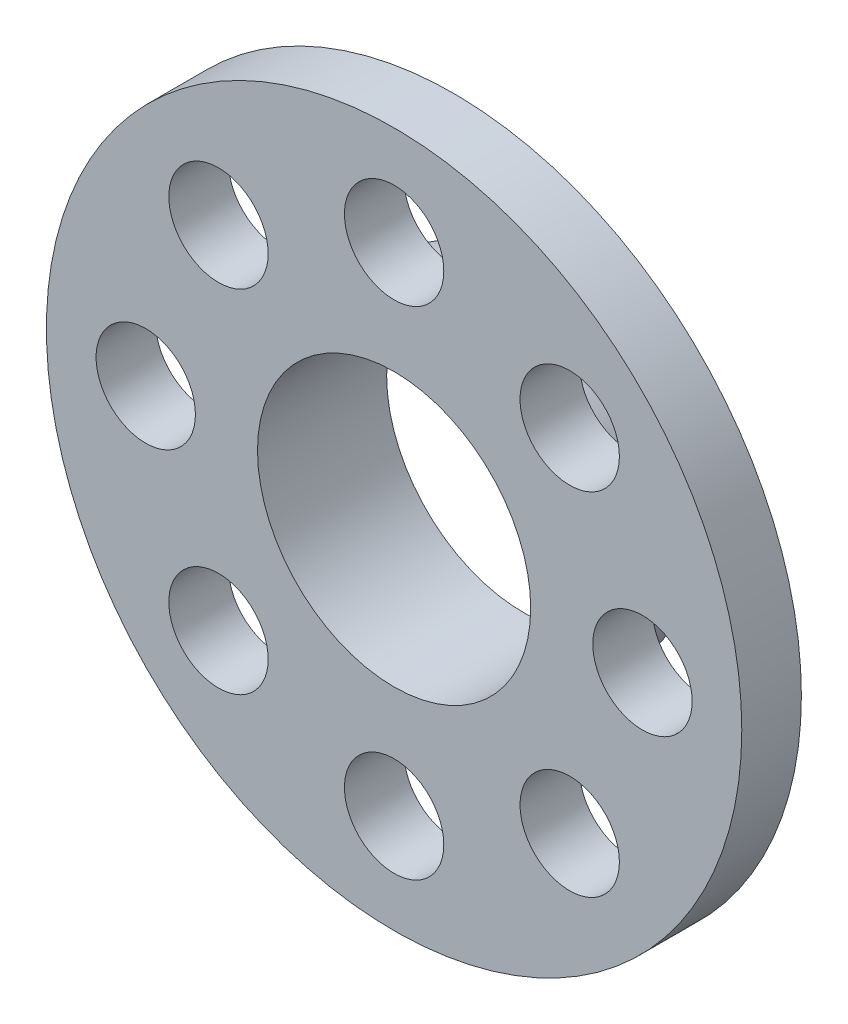
SolidWorks part; units mm, degrees
ref_plane "Front Plane" through (0, 0, 0) normal (0, 0, 1) x (1, 0, 0)
ref_plane "Top Plane" through (0, 0, 0) normal (0, 1, 0) x (1, 0, 0)
ref_plane "Right Plane" through (0, 0, 0) normal (1, 0, 0) x (0, 0, -1)
other "Configuration Table"
sketch "Sketch2" plane through (0, 0, 0) normal (0, 0, 1) x (1, 0, 0)
  circle A0 centre (0, 0) radius 70
  circle A1 centre (0, 0) radius 27.5
  dimension "D1" = 140
  dimension "D2" = 55
extrude "Boss-Extrude1" add sketch "Sketch2" along normal blind 12
sketch "Sketch3" plane through (0, 0, 12) normal (0, 0, 1) x (1, 0, 0)
  circle A0 centre (0, 0) radius 50 construction
  circle A1 centre (0, -50) radius 10
  dimension "D1" = 100
  dimension "D2" = 20
extrude "Cut-Extrude1" cut sketch "Sketch3" against normal through all both and the other way through all
pattern_circular "CirPattern1" count 8 over 360 about axis through (0, 0, 0) along (0, 0, 1) of "Cut-Extrude1"
sketch "Sketch4" plane through (0, 0, 0) normal (0, 0, -1) x (-1, 0, 0)
  circle A0 centre (0, 0) radius 33.5
  circle A1 centre (0, 0) radius 27.5 construction
  circle A2 centre (0, 0) radius 27.5
  dimension "D1" = 6
  dimension "D2" = 55
extrude "Boss-Extrude2" add sketch "Sketch4" along normal blind 14
